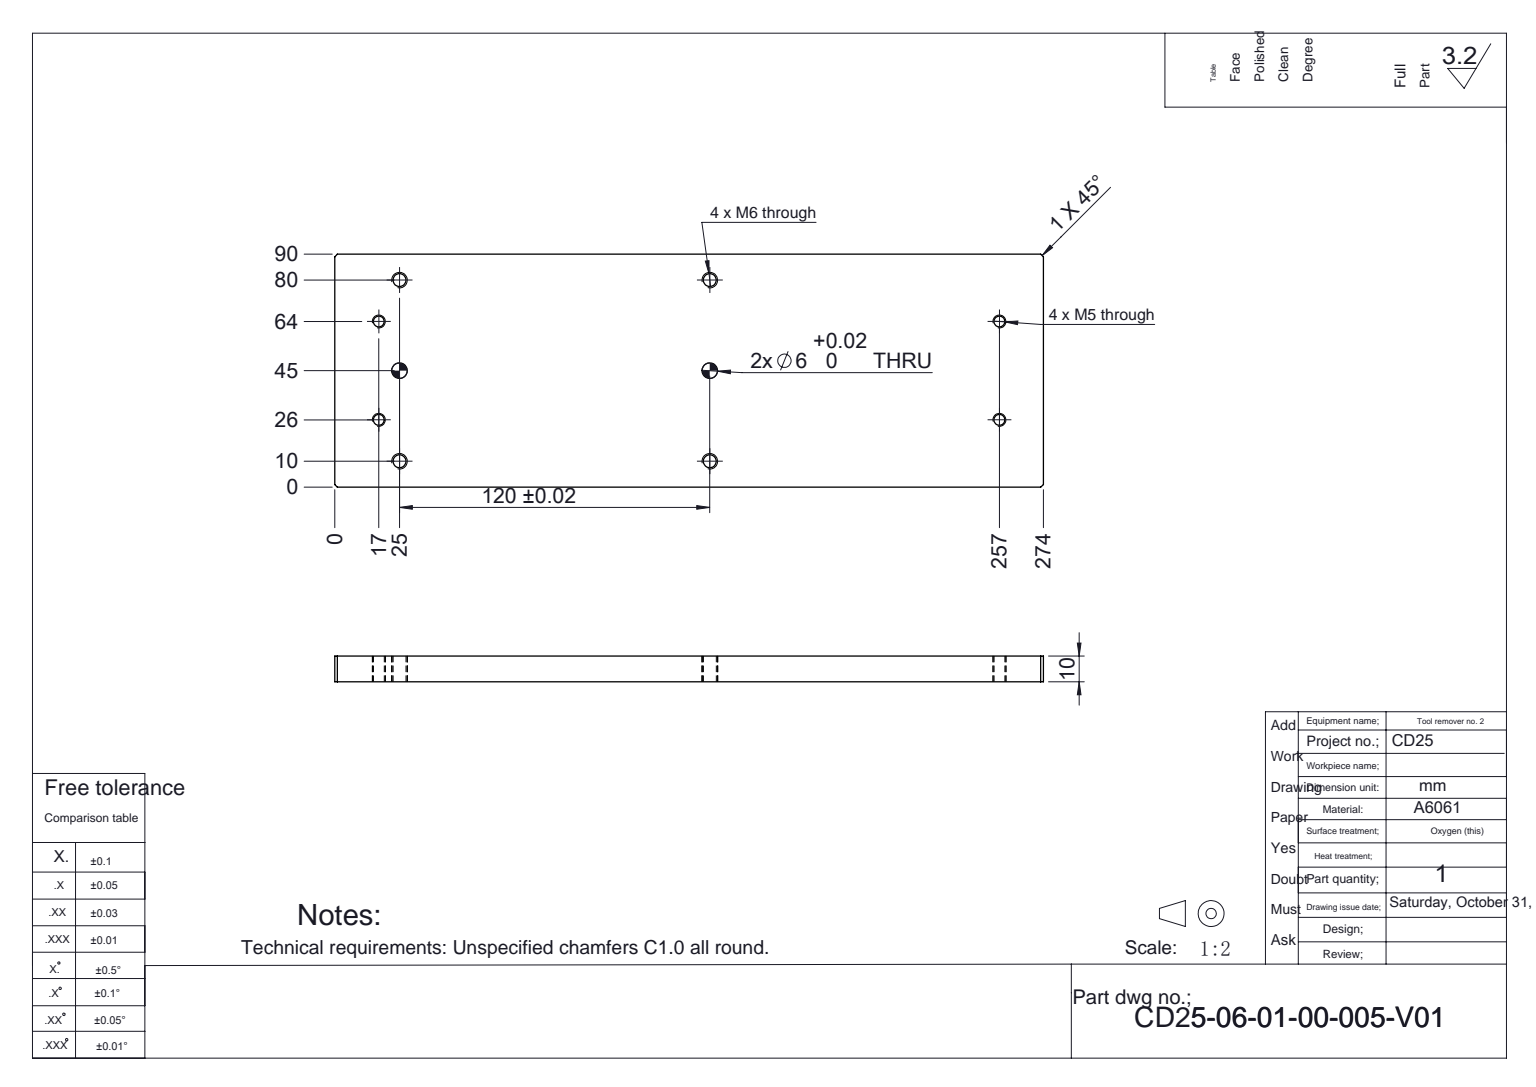
SolidWorks part; units mm, degrees
material "A6061"
ref_plane "Front Plane" through (0, 0, 0) normal (0, 0, 1) x (1, 0, 0)
ref_plane "Top Plane" through (0, 0, 0) normal (0, 1, 0) x (1, 0, 0)
ref_plane "Right Plane" through (0, 0, 0) normal (1, 0, 0) x (0, 0, -1)
sketch "Sketch1" plane through (0, 0, 0) normal (0, 0, 1) x (1, 0, 0)
  line L1 (-137, 45) -> (137, 45)
  line L2 (-137, 45) -> (-137, -45)
  line L3 (-137, -45) -> (137, -45)
  line L4 (137, 45) -> (137, -45)
  line L5 (-137, 45) -> (137, -45) construction
  line L6 (-137, -45) -> (137, 45) construction
  point P0 (0, 0)
  dimension "D1" = 274
  dimension "D2" = 90
extrude "Boss-Extrude1" add sketch "Sketch1" along normal mid plane 10
hole_wizard "M5 Tapped Hole1" positions "Sketch2" profile "Sketch3" tap size "M5" standard "GB" end condition through all
sketch "Sketch2" plane through (0, 0, 5) normal (0, 0, 1) x (1, 0, 0)
  point P0 (-120, 19)
  point P3 (-120, -19)
  point P6 (120, -19)
  point P9 (120, 19)
sketch "Sketch3" plane through (-120, 19, 5) normal (1, 0, 0) x (0, -1, 0)
  line L0 (0, 0) -> (0, 10)
  line L1 (0, 10) -> (2.1, 10)
  line L2 (2.1, 10) -> (2.1, 0)
  line L5 (2.1, 0) -> (0, 0)
  line L11 (0, -6.35) -> (0, 107.95) construction
  dimension "通孔螺纹孔钻头直径" = 4.2
  dimension "通孔螺纹孔钻头深度" = 10
cosmetic thread "Hole cosmetic thread1" parameters "D2"=5
cosmetic thread "Hole cosmetic thread2" parameters "D2"=5
cosmetic thread "Hole cosmetic thread3" parameters "D2"=5
cosmetic thread "Hole cosmetic thread4" parameters "D2"=5
hole_wizard "M6 Tapped Hole1" positions "Sketch4" profile "Sketch5" tap size "M6" standard "GB" end condition through all
sketch "Sketch4" plane through (0, 0, -5) normal (0, 0, -1) x (-1, 0, 0)
  point P0 (112, 35)
  point P3 (112, -35)
  point P6 (-8, -35)
  point P9 (-8, 35)
sketch "Sketch5" plane through (-112, 35, -5) normal (1, 0, 0) x (0, 1, 0)
  line L0 (0, 0) -> (0, 10)
  line L1 (0, 10) -> (2.5, 10)
  line L2 (2.5, 10) -> (2.5, 0)
  line L5 (2.5, 0) -> (0, 0)
  line L11 (0, -6.35) -> (0, 107.95) construction
  dimension "通孔螺纹孔钻头直径" = 5
  dimension "通孔螺纹孔钻头深度" = 10
cosmetic thread "Hole cosmetic thread5" parameters "D2"=6
cosmetic thread "Hole cosmetic thread6" parameters "D2"=6
cosmetic thread "Hole cosmetic thread7" parameters "D2"=6
cosmetic thread "Hole cosmetic thread8" parameters "D2"=6
hole_wizard "Ø6.0mm blind hole1" positions "Sketch6" profile "Sketch7" hole size "Ø6.0" standard "GB" end condition through all
sketch "Sketch6" plane through (0, 0, -5) normal (0, 0, -1) x (-1, 0, 0)
  point P0 (112, 0)
  point P3 (-8, 0)
sketch "Sketch7" plane through (-112, 0, -5) normal (1, 0, 0) x (0, 1, 0)
  line L0 (0, 0) -> (0, 10)
  line L1 (0, 10) -> (3, 10)
  line L2 (3, 10) -> (3, 0)
  line L5 (3, 0) -> (0, 0)
  line L11 (0, -6.35) -> (0, 107.95) construction
  dimension "通孔孔直径" = 6
  dimension "通孔孔深度" = 10
chamfer "Chamfer1" distance 1 angle 45 4 edges at (137, -45, 0) (-137, -45, 0) (-137, 45, 0) (137, 45, 0)
